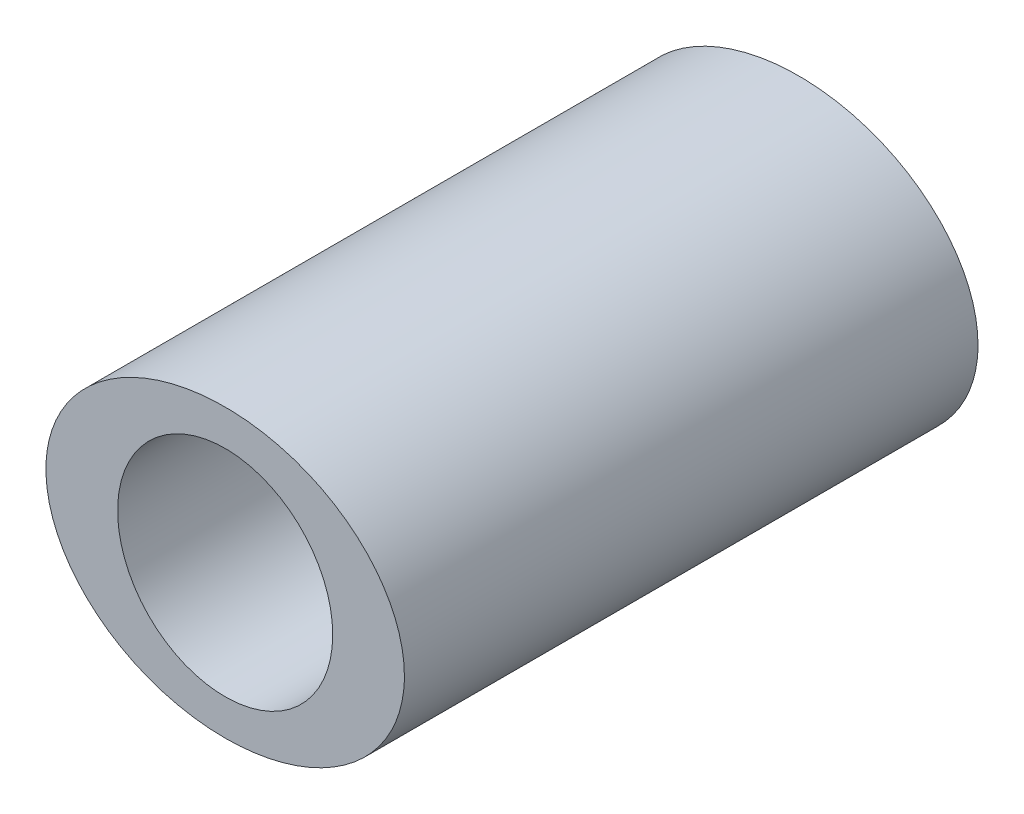
from build123d import *

# Parameters (mm, degrees)
SKETCH1_RX          = 25
SKETCH1_RY          = 20
BOSS_EXTRUDE1_DEPTH = 40
SKETCH2_R           = 15
CUT_EXTRUDE1_DEPTH  = 87.168439698


with BuildPart() as part:
    # Sketch1 → Boss-Extrude1 (new, symmetric)
    with BuildSketch(Plane.XY):
        with Locations((0, 0)):
            Ellipse(SKETCH1_RX, SKETCH1_RY)
    extrude(amount=BOSS_EXTRUDE1_DEPTH, both=True)

    # Sketch2 → Cut-Extrude1 (cut, through all)
    with BuildSketch(Plane.XY.offset(40)):
        Circle(SKETCH2_R)
    extrude(amount=-CUT_EXTRUDE1_DEPTH, mode=Mode.SUBTRACT)


solid = part.part
